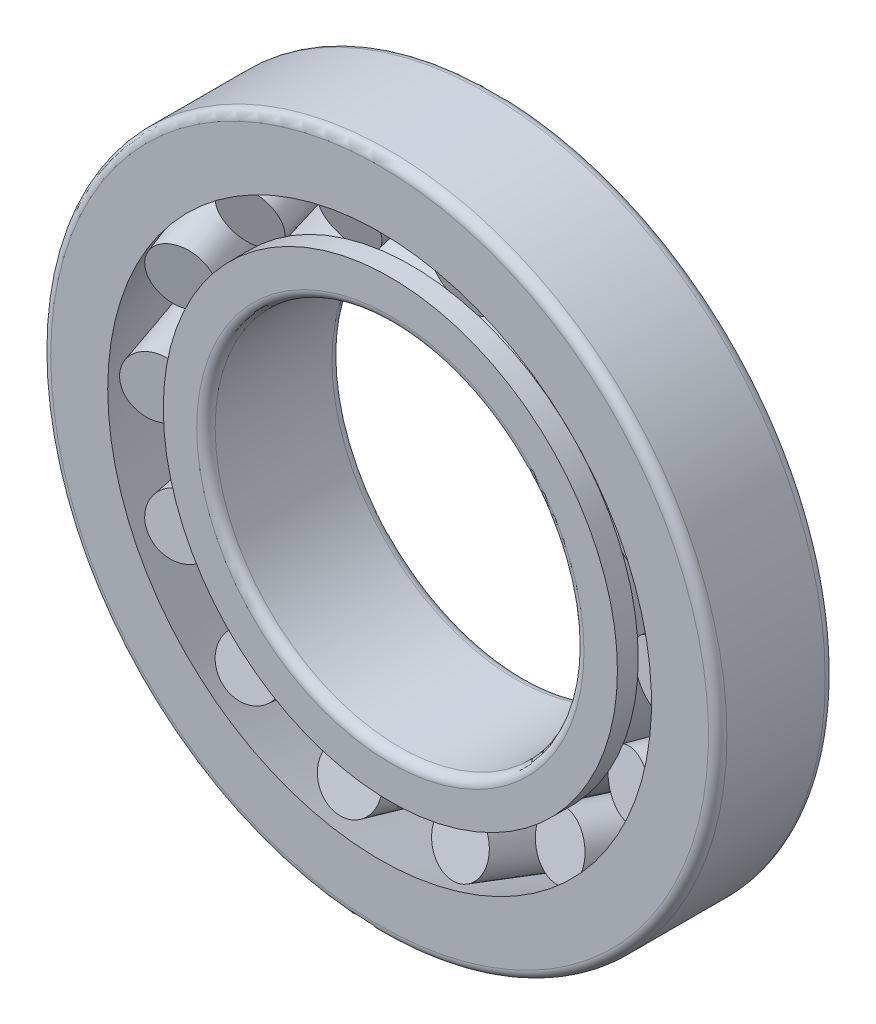
from build123d import *

# Parameters (mm, degrees)
PATTERN_CIRCULAR_1_COUNT = 14


with BuildPart() as part:
    # 草图1 → 旋转1 (revolve)
    with BuildSketch(Plane.XZ, mode=Mode.PRIVATE) as revolve_1_sk:
        with BuildLine():
            Line((40.599231026, 0), (31.5, 0))
            ThreePointArc((31.5, 0), (30.439339828, 0.439339828), (30, 1.5))
            Line((30, 1.5), (30, 20.5))
            ThreePointArc((30, 20.5), (30.439339828, 21.560660172), (31.5, 22))
            Line((31.5, 22), (36.940417606, 22))
            Line((36.940417606, 22), (36.940417606, 18.614664842))
            Line((36.940417606, 18.614664842), (35.743151795, 18.25276404))
            Line((35.743151795, 18.25276404), (39.401965215, 4.471948303))
            Line((39.401965215, 4.471948303), (40.599231026, 4.833849105))
            Line((40.599231026, 4.833849105), (40.599231026, 0))
        make_face()
    revolve(revolve_1_sk.sketch.rotate(Axis((0, 0, 0), (0, 0, 1)), 180), axis=Axis((0, 0, 0), (0, 0, 1)))


with BuildPart() as body_2:
    # 草图2 → 旋转2 (revolve)
    with BuildSketch(Plane(origin=(42.5, 0, 12.846590909), x_dir=(0, -1, 0), z_dir=(-0.9572254408742195, 0, -0.28934314462789035)), mode=Mode.PRIVATE) as revolve_2_sk:
        Polygon((0, -7.05375), (5.294963012, -7.05375), (4.805036988, 7.05375), (0, 7.05375), align=None)
    revolve(revolve_2_sk.sketch.rotate(Axis((42.5, 0, 12.846590909), (-0.2893431446278901, 0, 0.9572254408742195)), 270), axis=Axis((42.5, 0, 12.846590909), (-0.2893431446278901, 0, 0.9572254408742195)))


with BuildPart() as body_3:
    # 草图3 → 旋转3 (revolve)
    with BuildSketch(Plane.XZ, mode=Mode.PRIVATE) as revolve_3_sk:
        with BuildLine():
            Line((50.681917458, 4.75), (53.499999996, 4.75))
            ThreePointArc((53.499999996, 4.75), (54.560660168, 5.189339828), (54.999999996, 6.25))
            Line((54.999999996, 6.25), (54.999999996, 22.25))
            ThreePointArc((54.999999996, 22.25), (54.560660168, 23.310660172), (53.499999996, 23.75))
            Line((53.499999996, 23.75), (44.225535831, 23.75))
            Line((44.225535831, 23.75), (50.681917458, 4.75))
        make_face()
    revolve(revolve_3_sk.sketch.rotate(Axis((-4e-09, 0, 0), (0, 0, 1)), 180), axis=Axis((-4e-09, 0, 0), (0, 0, 1)))


with BuildPart() as pattern_circular_1_1:
    # 阵列(圆周)1: pattern copy
    add(body_2.part.rotate(Axis((0, 0, 0), (0, 0, 1)), 1 * 360 / PATTERN_CIRCULAR_1_COUNT))


with BuildPart() as pattern_circular_1_2:
    # 阵列(圆周)1: pattern copy
    add(body_2.part.rotate(Axis((0, 0, 0), (0, 0, 1)), 2 * 360 / PATTERN_CIRCULAR_1_COUNT))


with BuildPart() as pattern_circular_1_3:
    # 阵列(圆周)1: pattern copy
    add(body_2.part.rotate(Axis((0, 0, 0), (0, 0, 1)), 3 * 360 / PATTERN_CIRCULAR_1_COUNT))


with BuildPart() as pattern_circular_1_4:
    # 阵列(圆周)1: pattern copy
    add(body_2.part.rotate(Axis((0, 0, 0), (0, 0, 1)), 4 * 360 / PATTERN_CIRCULAR_1_COUNT))


with BuildPart() as pattern_circular_1_5:
    # 阵列(圆周)1: pattern copy
    add(body_2.part.rotate(Axis((0, 0, 0), (0, 0, 1)), 5 * 360 / PATTERN_CIRCULAR_1_COUNT))


with BuildPart() as pattern_circular_1_6:
    # 阵列(圆周)1: pattern copy
    add(body_2.part.rotate(Axis((0, 0, 0), (0, 0, 1)), 6 * 360 / PATTERN_CIRCULAR_1_COUNT))


with BuildPart() as pattern_circular_1_7:
    # 阵列(圆周)1: pattern copy
    add(body_2.part.rotate(Axis((0, 0, 0), (0, 0, 1)), 7 * 360 / PATTERN_CIRCULAR_1_COUNT))


with BuildPart() as pattern_circular_1_8:
    # 阵列(圆周)1: pattern copy
    add(body_2.part.rotate(Axis((0, 0, 0), (0, 0, 1)), 8 * 360 / PATTERN_CIRCULAR_1_COUNT))


with BuildPart() as pattern_circular_1_9:
    # 阵列(圆周)1: pattern copy
    add(body_2.part.rotate(Axis((0, 0, 0), (0, 0, 1)), 9 * 360 / PATTERN_CIRCULAR_1_COUNT))


with BuildPart() as pattern_circular_1_10:
    # 阵列(圆周)1: pattern copy
    add(body_2.part.rotate(Axis((0, 0, 0), (0, 0, 1)), 10 * 360 / PATTERN_CIRCULAR_1_COUNT))


with BuildPart() as pattern_circular_1_11:
    # 阵列(圆周)1: pattern copy
    add(body_2.part.rotate(Axis((0, 0, 0), (0, 0, 1)), 11 * 360 / PATTERN_CIRCULAR_1_COUNT))


with BuildPart() as pattern_circular_1_12:
    # 阵列(圆周)1: pattern copy
    add(body_2.part.rotate(Axis((0, 0, 0), (0, 0, 1)), 12 * 360 / PATTERN_CIRCULAR_1_COUNT))


with BuildPart() as pattern_circular_1_13:
    # 阵列(圆周)1: pattern copy
    add(body_2.part.rotate(Axis((0, 0, 0), (0, 0, 1)), 13 * 360 / PATTERN_CIRCULAR_1_COUNT))


solid = Compound([part.part, body_2.part, body_3.part, pattern_circular_1_1.part, pattern_circular_1_2.part, pattern_circular_1_3.part, pattern_circular_1_4.part, pattern_circular_1_5.part, pattern_circular_1_6.part, pattern_circular_1_7.part, pattern_circular_1_8.part, pattern_circular_1_9.part, pattern_circular_1_10.part, pattern_circular_1_11.part, pattern_circular_1_12.part, pattern_circular_1_13.part])
